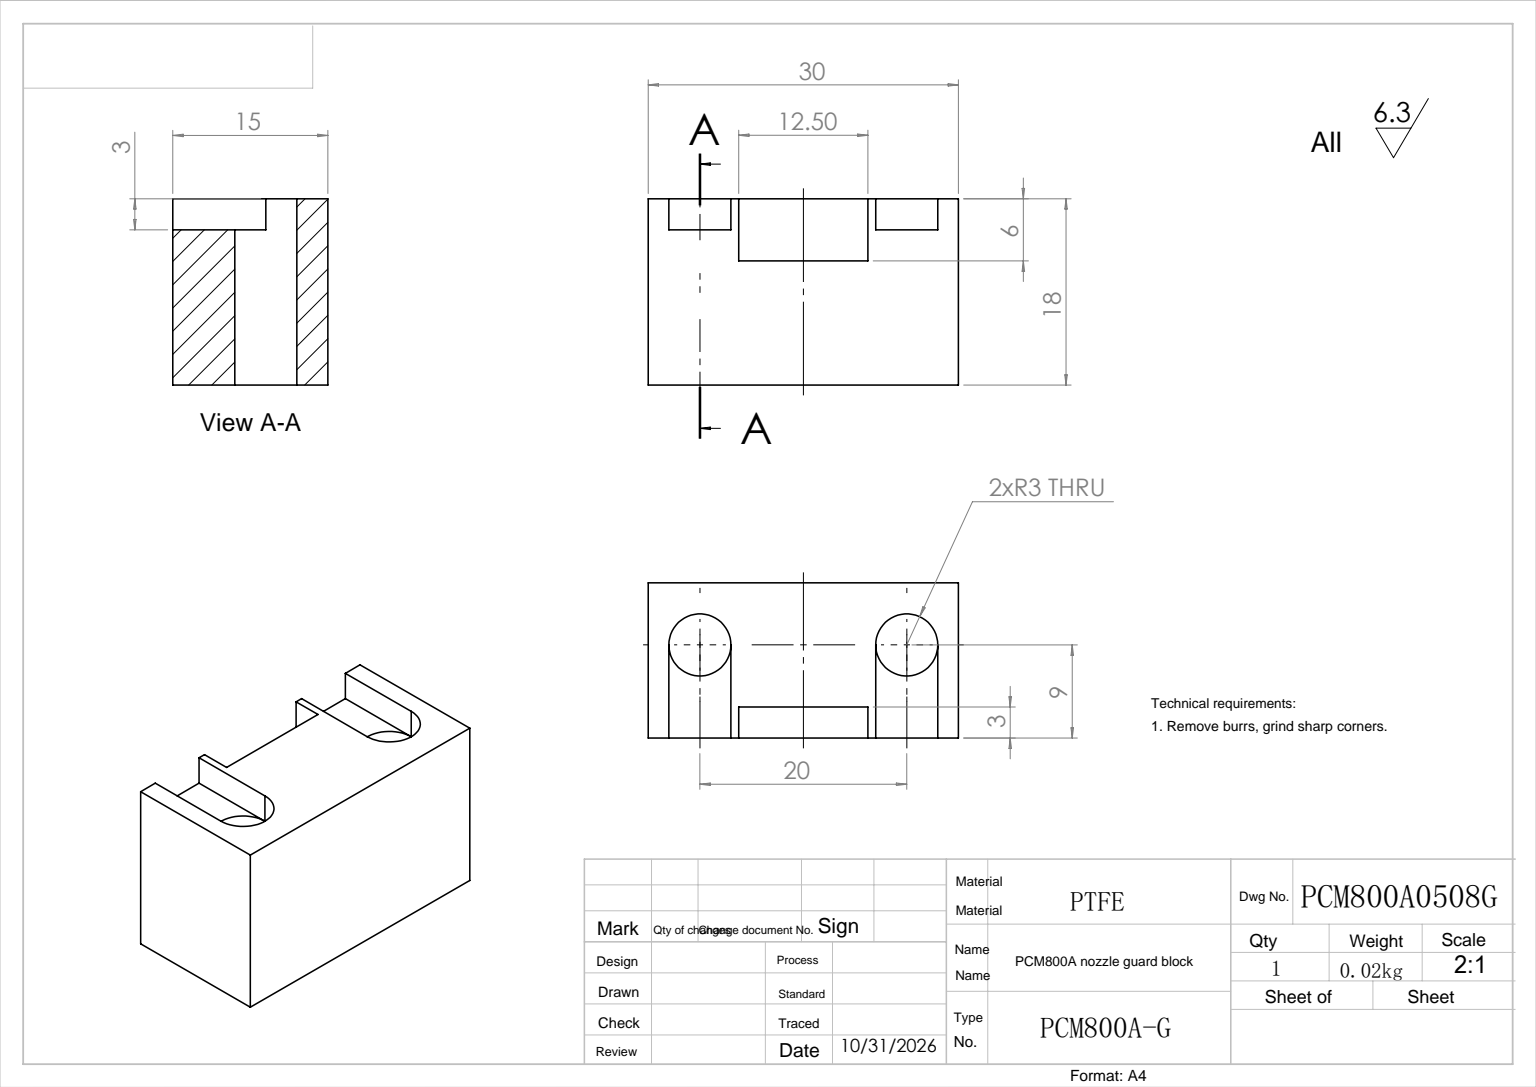
SolidWorks part; units mm, degrees
ref_plane "前视基准面" through (0, 0, 0) normal (0, 0, 1) x (1, 0, 0)
ref_plane "上视基准面" through (0, 0, 0) normal (0, 1, 0) x (1, 0, 0)
ref_plane "右视基准面" through (0, 0, 0) normal (1, 0, 0) x (0, 0, -1)
sketch "草图1" plane through (0, 0, 0) normal (0, 0, 1) x (1, 0, 0)
  line L1 (0, 0) -> (15, 0)
  line L2 (0, 0) -> (0, 18)
  line L3 (0, 18) -> (15, 18)
  line L4 (15, 0) -> (15, 18)
  dimension "D1" = 18
  dimension "D2" = 15
extrude "拉伸1" add sketch "草图1" along normal blind 30
sketch "草图2" plane through (0, 18, 0) normal (0, 1, 0) x (-1, 0, 0)
  line L0 (0, 5) -> (-13.4158, 5) construction
  line L1 (0, 30) -> (0, 0) construction
  line L2 (-15, 0) -> (0, 0) construction
  circle A0 centre (-6, 5) radius 3
  dimension "D1" = 6
  dimension "D2" = 6
  dimension "D3" = 5
extrude "切除-拉伸1" cut sketch "草图2" against normal through all
sketch "草图4" plane through (0, 18, 0) normal (0, 1, 0) x (-1, 0, 0)
  line L0 (-15, 2) -> (-6, 2)
  line L1 (-15, 15) -> (1.9157, 15) construction
  line L2 (-15, 30) -> (-15, 0) construction
  line L3 (-15, 8) -> (-6, 8)
  line L4 (-15, 2) -> (-15, 8)
  arc A0 (-6, 2) -> (-6, 8) centre (-6, 5) ccw
  circle A1 centre (-6, 5) radius 3 construction
  dimension "D1" = 6
extrude "切除-拉伸3" cut sketch "草图4" against normal blind 3
pattern_linear "阵列(线性)1" count 2 spacing 20 along (0, 0, 1) of "切除-拉伸3", "切除-拉伸1"
sketch "草图5" plane through (15, 3, 0) normal (-1, 0, 0) x (0, 1, 0)
  line L0 (15, -22) -> (15, -8) construction
  line L1 (9, -21.25) -> (15, -21.25)
  line L2 (9, -21.25) -> (9, -8.75)
  line L3 (9, -8.75) -> (15, -8.75)
  line L4 (15, -21.25) -> (15, -8.75)
  line L5 (-3, -30) -> (15, -30) construction
  dimension "D1" = 12.5
  dimension "D2" = 6
  dimension "D3" = 8.75
extrude "切除-拉伸4" cut sketch "草图5" along normal blind 3
